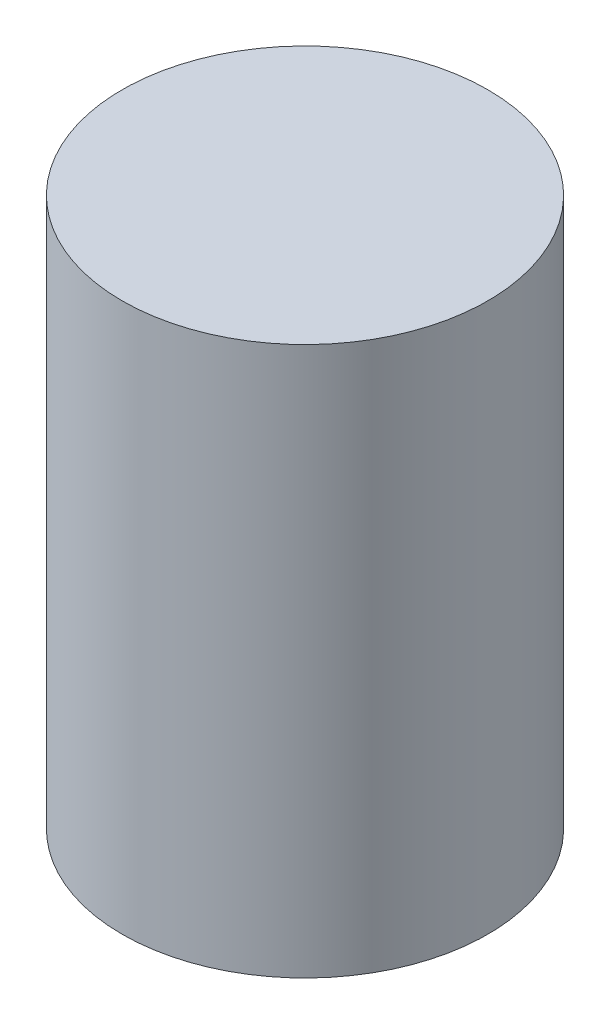
SolidWorks part; units mm, degrees
ref_plane "Front Plane" through (0, 0, 0) normal (0, 0, 1) x (1, 0, 0)
ref_plane "Top Plane" through (0, 0, 0) normal (0, 1, 0) x (1, 0, 0)
ref_plane "Right Plane" through (0, 0, 0) normal (1, 0, 0) x (0, 0, -1)
sketch "Sketch1" plane through (0, 0, 0) normal (0, 1, 0) x (1, 0, 0)
  circle A0 centre (0, 0) radius 10
  dimension "D1" = 20
extrude "Boss-Extrude1" add sketch "Sketch1" along normal blind 30
